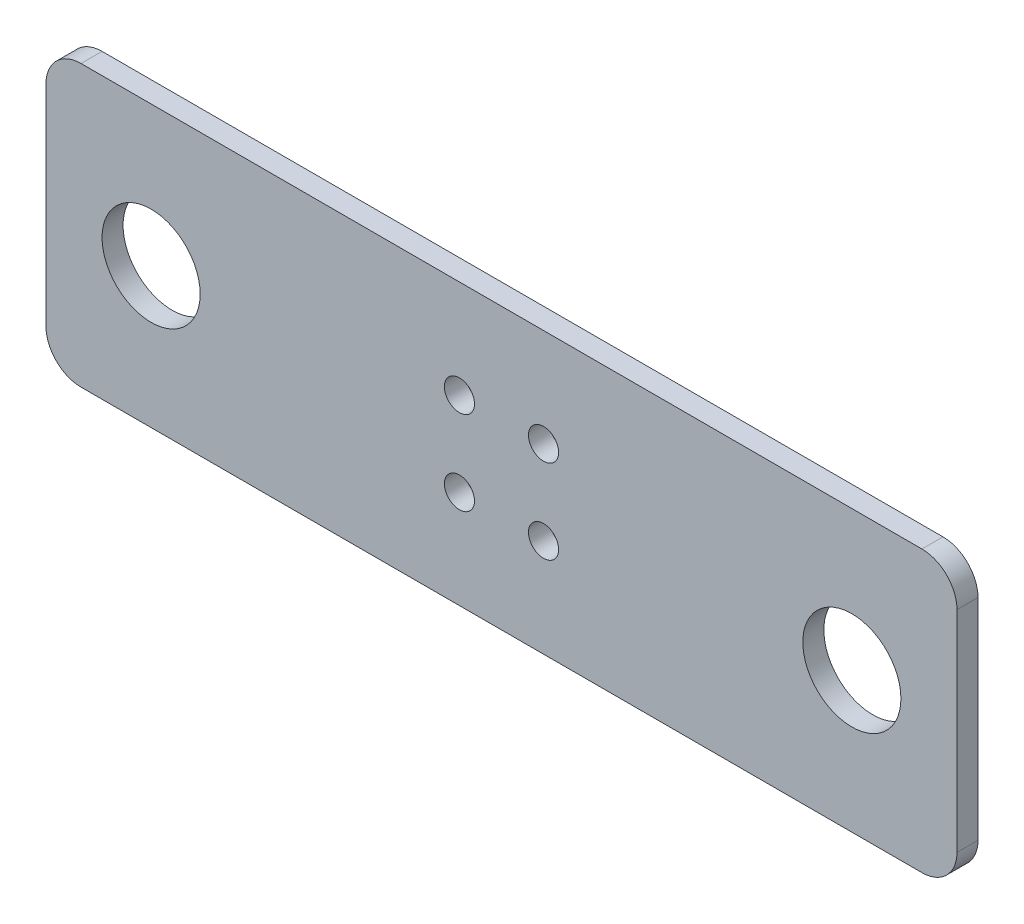
SolidWorks part; units mm, degrees
ref_plane "前视基准面" through (0, 0, 0) normal (0, 0, 1) x (1, 0, 0)
ref_plane "上视基准面" through (0, 0, 0) normal (0, 1, 0) x (1, 0, 0)
ref_plane "右视基准面" through (0, 0, 0) normal (1, 0, 0) x (0, 0, -1)
sketch "草图1" plane through (0, 0, 0) normal (0, 0, 1) x (1, 0, 0)
  line L1 (-65, 20) -> (65, 20)
  line L2 (-65, 20) -> (-65, -20)
  line L3 (-65, -20) -> (65, -20)
  line L4 (65, 20) -> (65, -20)
  line L5 (-65, 20) -> (65, -20) construction
  line L6 (-65, -20) -> (65, 20) construction
  point P0 (0, 0)
  dimension "D1" = 130
  dimension "D2" = 40
extrude "凸台-拉伸1" add sketch "草图1" along normal blind 3
sketch "草图2" plane through (0, 0, 3) normal (0, 0, 1) x (1, 0, 0)
  line L0 (-50, 0) -> (0, 0) construction
  line L1 (0, 0) -> (50, 0) construction
  line L3 (-6, 6) -> (6, 6) construction
  line L4 (-6, 6) -> (-6, -6) construction
  line L5 (-6, -6) -> (6, -6) construction
  line L6 (6, 6) -> (6, -6) construction
  line L7 (-6, 6) -> (6, -6) construction
  line L8 (-6, -6) -> (6, 6) construction
  circle A0 centre (-50, 0) radius 7
  circle A1 centre (50, 0) radius 7
  circle A2 centre (-6, 6) radius 2.15
  circle A3 centre (6, 6) radius 2.15
  circle A4 centre (6, -6) radius 2.15
  circle A5 centre (-6, -6) radius 2.15
  dimension "D2" = 14
  dimension "D4" = 4.3
  dimension "D1" = 100
  dimension "D3" = 12
extrude "切除-拉伸1" cut sketch "草图2" against normal blind 3
fillet "圆角1" radius 5 4 edges at (65, 20, 1.5) (65, -20, 1.5) (-65, 20, 1.5) (-65, -20, 1.5)
